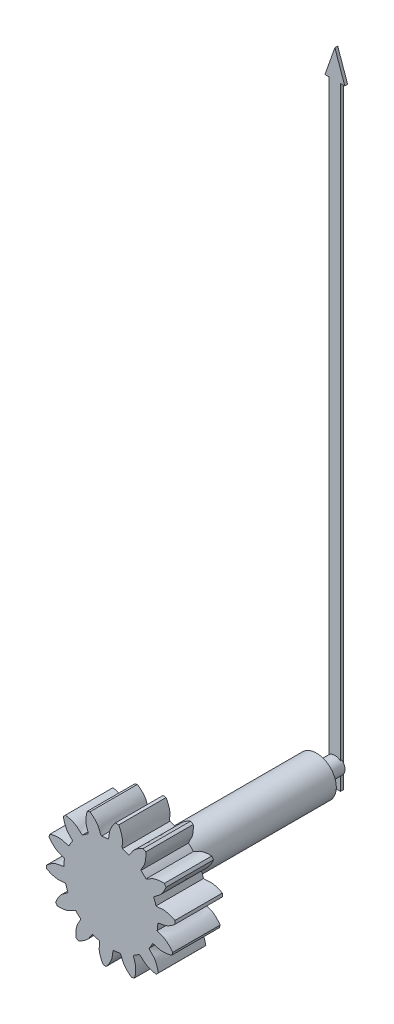
SolidWorks part; units mm, degrees
ref_plane "Front Plane" through (0, 0, 0) normal (0, 0, 1) x (1, 0, 0)
ref_plane "Top Plane" through (0, 0, 0) normal (0, 1, 0) x (1, 0, 0)
ref_plane "Right Plane" through (0, 0, 0) normal (1, 0, 0) x (0, 0, -1)
sketch "Sketch1" plane through (0, 0, 0) normal (0, 0, 1) x (1, 0, 0)
  circle A0 centre (0, 0) radius 1.188
  circle A1 centre (0, 0) radius 0.5
extrude "Boss-Extrude1" add sketch "Sketch1" along normal blind 1.2
sketch "Sketch2" plane through (0, 0, 0) normal (0, 0, 1) x (1, 0, 0)
  arc A0 (1.6194, 0.2458) -> (1.6292, 0.1693) centre (0, 0) cw
  arc A1 (1.1426, 0.3252) -> (1.1877, -0.0274) centre (0, 0) cw
  spline S0 degree 3 poles (1.6292, 0.1693) (1.5913, 0.1347) (1.5316, 0.0876) (1.4455, 0.0395) (1.3415, -0.0059) (1.2488, -0.0032) (1.1877, -0.0274) knots 0 0 0 0 0.313167 0.460103 0.600583 1 1 1 1
  spline S1 degree 3 poles (1.6194, 0.2458) (1.574, 0.2698) (1.5044, 0.3004) (1.409, 0.3252) (1.2969, 0.3431) (1.2079, 0.3171) (1.1426, 0.3252) knots 0 0 0 0 0.313167 0.460103 0.600583 1 1 1 1
extrude "Boss-Extrude2" add sketch "Sketch2" along normal blind 1.2
pattern_circular "CirPattern1" count 14 over 360 about axis through (0, 0, 1.2) along (0, 0, -1) of "Boss-Extrude2"
sketch "Sketch3" plane through (0, 0, 0) normal (0, 0, -1) x (-1, 0, 0)
  circle A0 centre (0, 0) radius 0.5
extrude "Boss-Extrude3" add sketch "Sketch3" along normal blind 4 and the other way blind 1.2
sketch "Sketch4" plane through (0, 0, -4) normal (0, 0, -1) x (-1, 0, 0)
  circle A0 centre (0, 0) radius 0.2194
extrude "Boss-Extrude4" add sketch "Sketch4" along normal blind 0.5
sketch "Sketch5" plane through (0, 0, 0) normal (0, 1, 0) x (1, 0, 0)
  line L0 (0.2194, 4.5) -> (-0.2194, 4.5) construction
  line L1 (0.1422, 4.4637) -> (-0.1422, 4.4637)
  line L2 (0.1422, 4.4637) -> (0.1422, 4.5363)
  line L3 (0.1422, 4.5363) -> (-0.1422, 4.5363)
  line L4 (-0.1422, 4.4637) -> (-0.1422, 4.5363)
  line L5 (0, 4.5363) -> (0, 4.4637) construction
  line L6 (0.1422, 4.5) -> (-0.1422, 4.5) construction
  point P0 (0, 4.5)
extrude "Boss-Extrude5" add sketch "Sketch5" along normal blind 15 and the other way blind 0.5
sketch "Sketch6" plane through (0, 0, -4.5363) normal (0, 0, -1) x (-1, 0, 0)
  line L0 (0, 15) -> (-0.25, 15)
  line L1 (-0.1422, 15) -> (0.1422, 15) construction
  line L2 (-0.25, 15) -> (0, 15.713)
  line L3 (0, 15.713) -> (0.25, 15)
  line L4 (0.25, 15) -> (0, 15)
  dimension "D1" = 0.25
  dimension "D2" = 0.25
extrude "Boss-Extrude6" add sketch "Sketch6" against normal up to surface (0.0727 mm away) up to face at (0, 7.5966, -4.4637)
